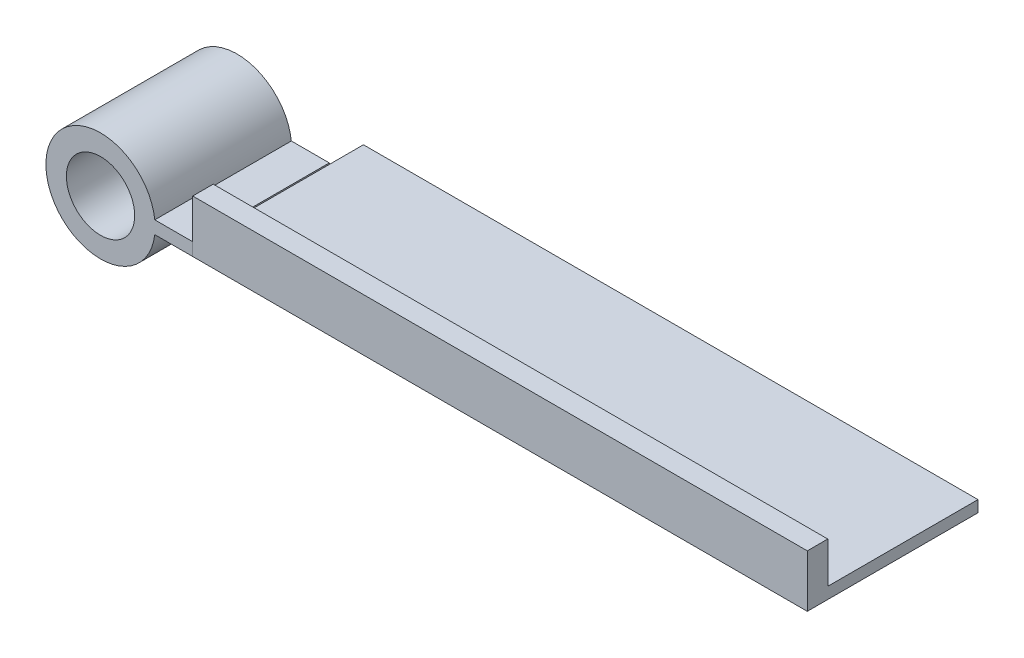
from build123d import *

# Parameters (mm, degrees)
SKETCH1_R           = 8
SKETCH1_R_2         = 5
BOSS_EXTRUDE1_DEPTH = 10
SKETCH3_W           = 8
SKETCH3_H           = 1.874989596
BOSS_EXTRUDE2_DEPTH = 10
SKETCH4_W           = 90
SKETCH4_H           = 7.675222422
BOSS_EXTRUDE3_DEPTH = 25
SKETCH5_W           = 90
SKETCH5_H           = 22
CUT_EXTRUDE1_DEPTH  = 6


with BuildPart() as part:
    # Sketch1 → Boss-Extrude1 (new, symmetric)
    with BuildSketch(Plane.XY):
        Circle(SKETCH1_R)
        Circle(SKETCH1_R_2, mode=Mode.SUBTRACT)
    extrude(amount=BOSS_EXTRUDE1_DEPTH, both=True)

    # Sketch3 → Boss-Extrude2 (add, symmetric)
    with BuildSketch(Plane.XY):
        with Locations((9.5, 0)):
            Rectangle(SKETCH3_W, SKETCH3_H)
    extrude(amount=BOSS_EXTRUDE2_DEPTH, both=True)


with BuildPart() as body_2:
    # Sketch4 → Boss-Extrude3 (new body)
    with BuildSketch(Plane.XY.offset(10)):
        with Locations((58.5, 2.900116413)):
            Rectangle(SKETCH4_W, SKETCH4_H)
    extrude(amount=-BOSS_EXTRUDE3_DEPTH)

    # Sketch5 → Cut-Extrude1 (cut)
    with BuildSketch(Plane(origin=(0, 6.737727624, 0), x_dir=(1, 0, 0), z_dir=(0, 1, 0))):
        with Locations((58.5, 4)):
            Rectangle(SKETCH5_W, SKETCH5_H)
    extrude(amount=-CUT_EXTRUDE1_DEPTH, mode=Mode.SUBTRACT)


solid = Compound([part.part, body_2.part])
